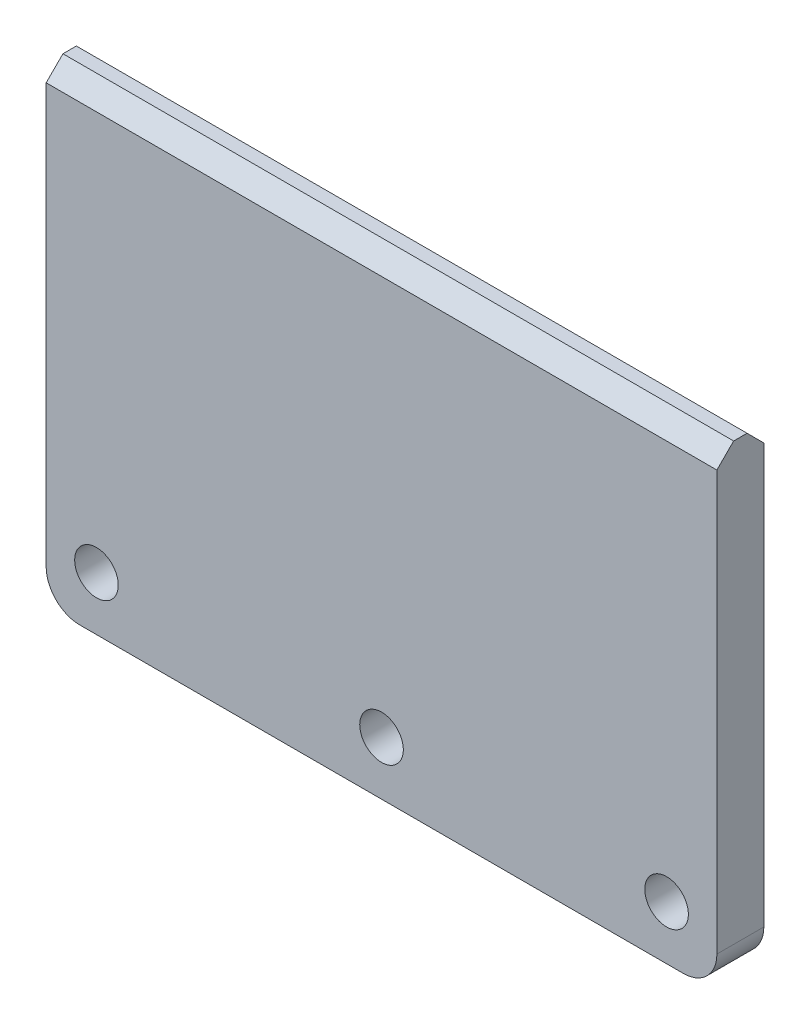
SolidWorks part; units mm, degrees
material "普通碳钢"
ref_plane "Front Plane" through (0, 0, 0) normal (0, 0, 1) x (1, 0, 0)
ref_plane "Top Plane" through (0, 0, 0) normal (0, 1, 0) x (1, 0, 0)
ref_plane "Right Plane" through (0, 0, 0) normal (1, 0, 0) x (0, 0, -1)
sketch "Sketch1" plane through (0, 0, 0) normal (0, 0, 1) x (1, 0, 0)
  line L1 (0, 0) -> (200, 0)
  line L2 (0, 0) -> (0, 140)
  line L3 (0, 140) -> (200, 140)
  line L4 (200, 0) -> (200, 140)
  dimension "D1" = 140
  dimension "D2" = 200
extrude "Boss-Extrude1" add sketch "Sketch1" along normal blind 14
chamfer "Chamfer1" distance 5 angle 45 2 edges at (100, 140, 14) (100, 140, 0)
sketch "Sketch2" plane through (0, 0, 0) normal (0, 0, -1) x (-1, 0, 0)
  line L0 (-175, 17.5) -> (-125, 17.5) construction
  line L1 (-125, 17.5) -> (-75, 17.5) construction
  line L2 (-75, 17.5) -> (-25, 17.5) construction
  line L3 (-100, 17.5) -> (-100, 0) construction
  line L4 (0, 0) -> (-200, 0) construction
  circle A0 centre (-175, 17.5) radius 6.5
  circle A1 centre (-125, 17.5) radius 6.5
  circle A2 centre (-75, 17.5) radius 6.5
  circle A3 centre (-25, 17.5) radius 6.5
  dimension "D3" = 13
  dimension "D1" = 17.5
  dimension "D2" = 50
extrude "Cut-Extrude1" [suppressed] cut sketch "Sketch2" against normal through all
sketch "Sketch3" plane through (0, 0, 0) normal (0, 0, -1) x (-1, 0, 0)
  line L0 (-185, 16) -> (-100, 16) construction
  line L1 (-100, 16) -> (-15, 16) construction
  line L2 (-100, 16) -> (-100, 0) construction
  line L3 (0, 0) -> (-200, 0) construction
  circle A0 centre (-185, 16) radius 6.5
  circle A1 centre (-100, 16) radius 6.5
  circle A2 centre (-15, 16) radius 6.5
  dimension "D2" = 13
  dimension "D1" = 16
  dimension "D3" = 85
extrude "Cut-Extrude2" cut sketch "Sketch3" against normal through all
fillet "Fillet1" radius 10 2 edges at (200, 0, 7) (0, 0, 7)
